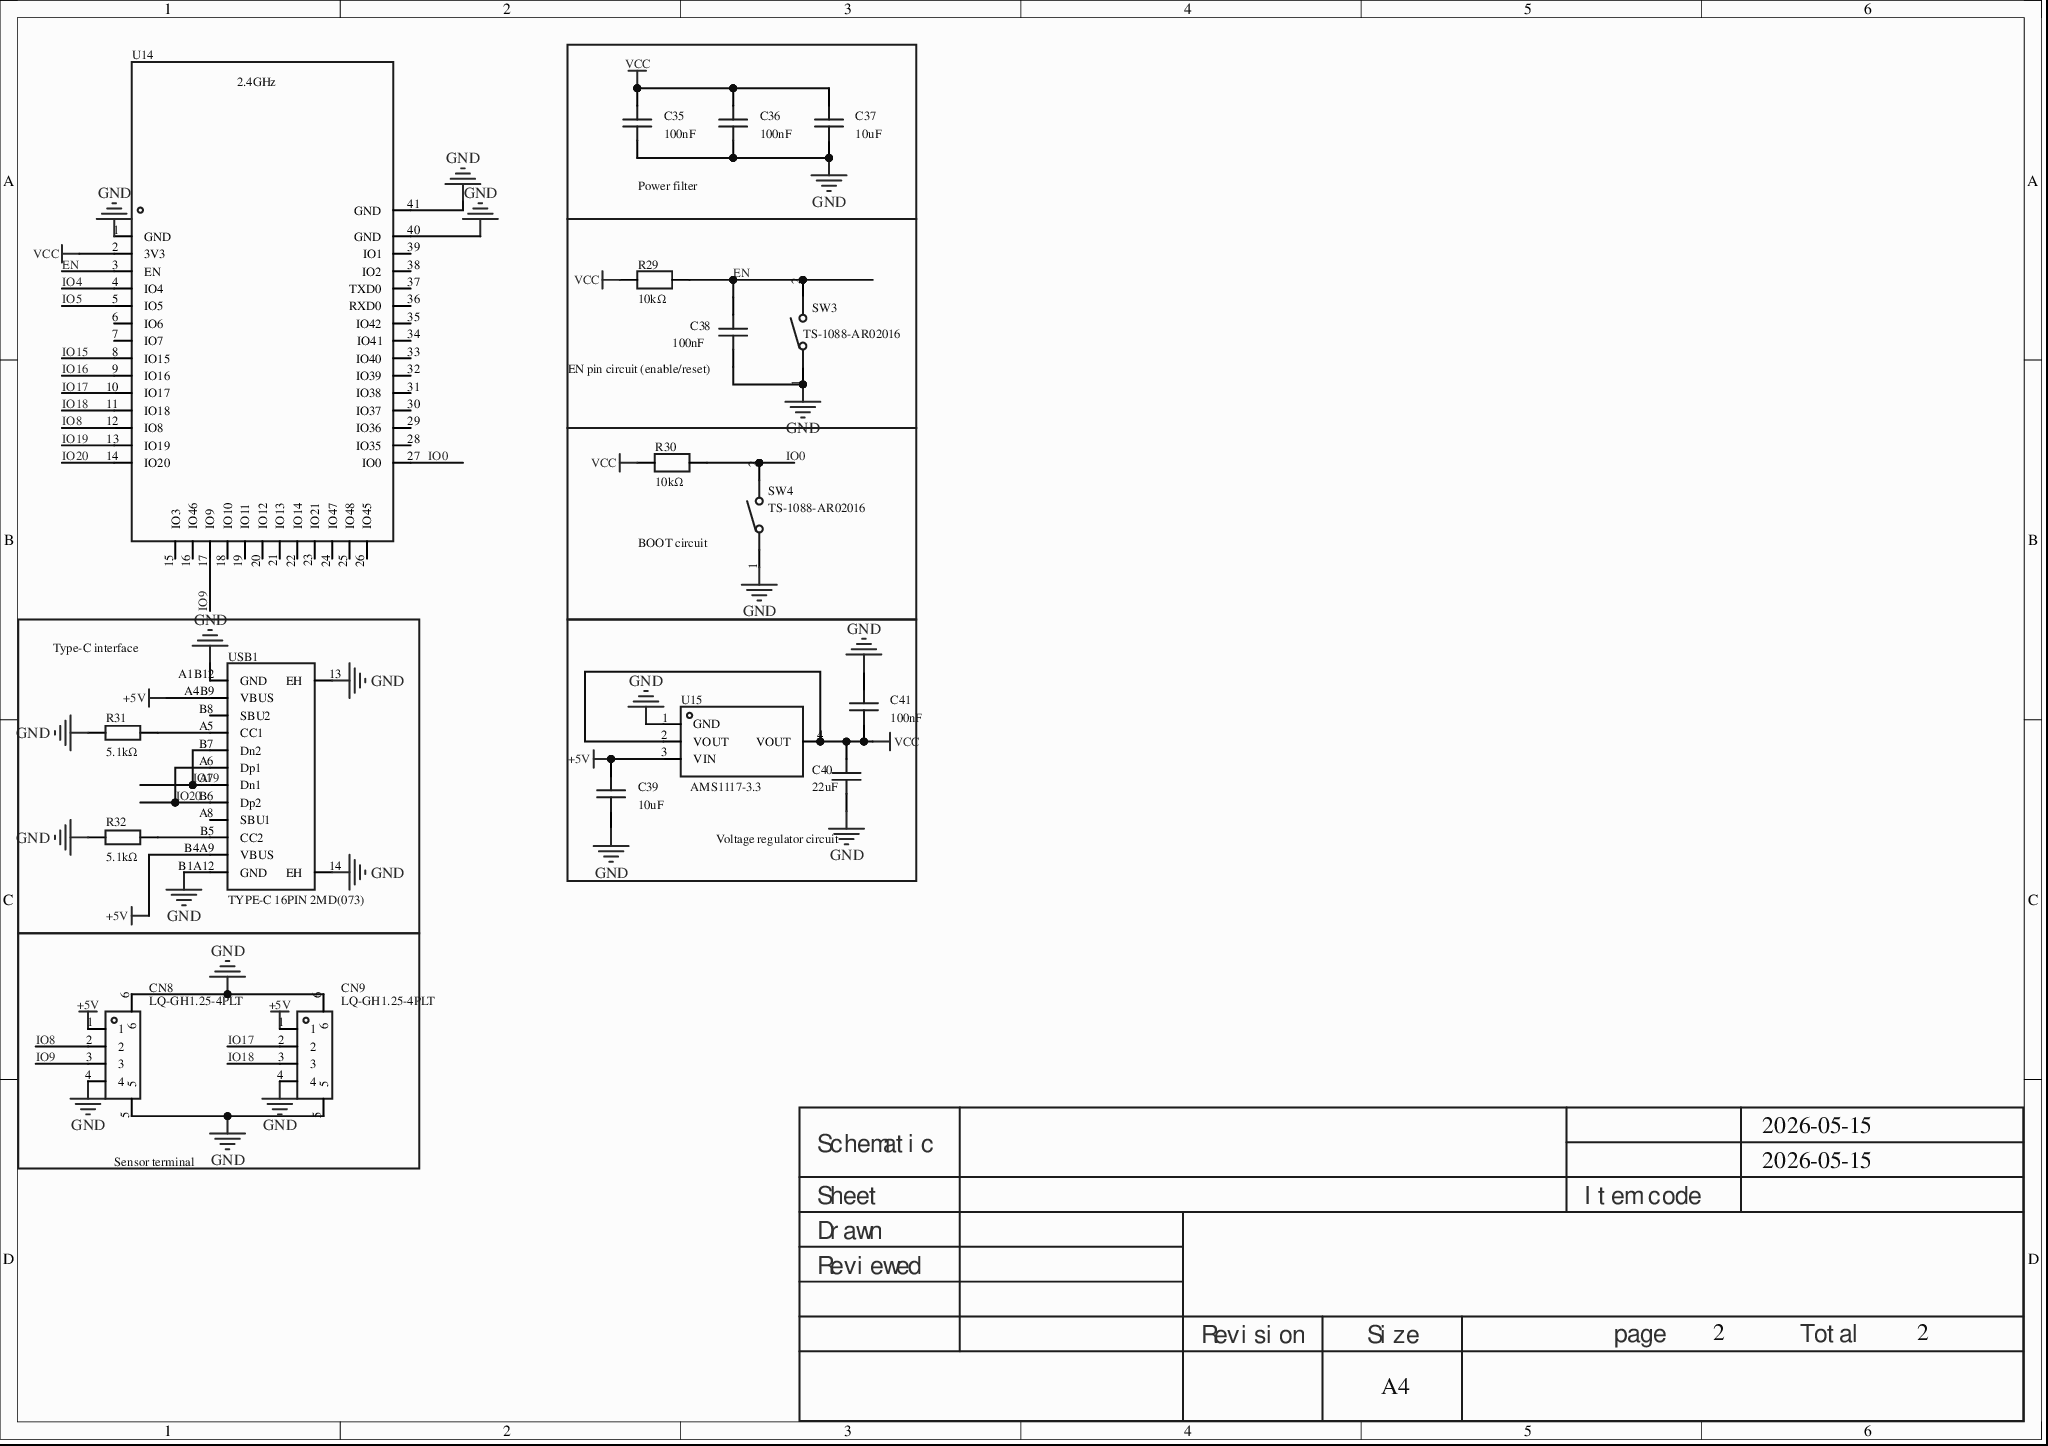
[diagram p0: MISC62500-3.schdoc]
# Altium project MISC62500-2.PrjPcb (part 1 of 2)
2 sheets, 106 parts. Net scope: global (net labels, ports and power ports of the same name join across sheets).
Board file: MISC62500.pcbdoc
Sheets:
  MISC62500-3.schdoc
  MISC62500-4.schdoc

## Sheet MISC62500-3.schdoc
size 297 x 209 mm; Version: V1.0; @Project Name: MISC62500; @Page Count: 2; @Update Date: 2026-05-15; @Create Date: 2026-05-15; @Schematic Name: MISC62500; @Page No: 2; @Board Name: MISC62500; @Create Time: 10:23:29; @Update Time: 19:47:53

### Parts
C35  100nF  [C0603]
C36  100nF  [C0603]
C37  10uF  [C0805]
C38  100nF  [C0603]
C39  10uF  [C0805]
C40  22uF  [C0805]
C41  100nF  [C0603]
CN8  LQ-GH1.25-4PLT  [CONN-SMD_LQ-GH1.25-4PLT]
CN9  LQ-GH1.25-4PLT  [CONN-SMD_LQ-GH1.25-4PLT]
R29  10kΩ  [R0603]
R30  10kΩ  [R0603]
R31  5.1kΩ  [R0603]
R32  5.1kΩ  [R0603]
SW3  TS-1088-AR02016  [SW-SMD_L3.9-W3.0-P4.45]
SW4  TS-1088-AR02016  [SW-SMD_L3.9-W3.0-P4.45]
U14  2.4GHz  [WIRELM-SMD_ESP32-S3-WROOM-1]
U15  AMS1117-3.3  [SOT-223-3_L6.5-W3.4-P2.30-LS7.0-BR]
USB1  TYPE-C 16PIN 2MD(073)  [USB-C-SMD_TYPE-C-16PIN-2MD-073]

### Blocks framed on the sheet
Power filter: C35-C37
EN pin circuit (enable/reset): C38 R29 SW3
BOOT circuit: R30 SW4
Type-C interface: R31 R32 USB1
Voltage regulator circuit: C39-C41 U15
Sensor terminal: CN8 CN9

### Nets
+5V: C39.2 CN8.1 CN9.1 U15.3(VIN) USB1.A4B9(VBUS) USB1.B4A9(VBUS)
GND: C35.1 C36.1 C37.1 C38.1 C39.1 C40.1 C41.2 CN8.4 CN8.5 CN8.6 CN9.4 CN9.5 CN9.6 R31.1 R32.1 SW3.1 SW4.1 U14.1(GND) U14.40(GND) U14.41(GND) U15.1(GND) USB1.13(EH) USB1.14(EH) USB1.A1B12(GND) USB1.B1A12(GND)
VCC: C35.2 C36.2 C37.2 C40.2 C41.1 R29.1 R30.1 U14.2(3V3) U15.2(VOUT) U15.4(VOUT)
EN: C38.2 R29.2 SW3.2 U14.3(EN)
IO0: R30.2 SW4.2 U14.27(IO0)
IO4: U14.4(IO4)
IO5: U14.5(IO5)
IO8: CN8.2 U14.12(IO8)
IO9: CN8.3 U14.17(IO9)
IO15: U14.8(IO15)
IO16: U14.9(IO16)
IO17: CN9.2 U14.10(IO17)
IO18: CN9.3 U14.11(IO18)
IO19: U14.13(IO19) USB1.A7(Dn1) USB1.B7(Dn2)
IO20: U14.14(IO20) USB1.A6(Dp1) USB1.B6(Dp2)
NetR31_2: R31.2 USB1.A5(CC1)
NetR32_2: R32.2 USB1.B5(CC2)

Not connected (* = marked no-connect by the designer): U14 6(IO6)* 7(IO7)* 15(IO3)* 16(IO46)* 18(IO10)* 19(IO11)* 20(IO12)* 21(IO13)* 22(IO14)* 23(IO21)* 24(IO47)* 25(IO48)* 26(IO45)* 28(IO35)* 29(IO36)* 30(IO37)* 31(IO38)* 32(IO39)* 33(IO40)* 34(IO41)* 35(IO42)* 36(RXD0)* 37(TXD0)* 38(IO2)* 39(IO1)*; USB1 A8(SBU1)* B8(SBU2)*

### Notes on the sheet
- 2026-05-15
- Schematic
- Sheet
- Item code
- Reviewed
- Drawn
- Revision
- Size
- A4
- page
- 2
- Total

### Library data of the parts
C35 C36 C38 C41 = CC0603KRX7R9BB104: Capacitance: 100nF; Tolerance: ±10%; Rated voltage: 50V; Temp coefficient: X7R;; Manufacturer: YAGEO(国巨); AddInBom: yes; ModelId: ac125912035d415993ca9572d50418b1; ModelName: C0603_L1.6-W0.8-H0.8; ModelTransform: 62.992,31.496,0,0,0,0,0,0,0; Symbol: CC0603KRX7R9BB104; Device: CC0603KRX7R9BB104; LCSC Part Name: 100nF ±10% 50V; SupplierPart: C14663; ManufacturerPart: CC0603KRX7R9BB104; Supplier Footprint: 0603; JLCPCB Part Class: Basic Part; Datasheet: example.com/datasheet/CC0603KRX7R9BB104/15331.html; Supplier: LCSC; ConvertToPcb: yes; FootprintName: C0603; Value: 100nF; Voltage Rating: 50V; Temperature Coefficient: X7R
C37 C39 = CGA0805X5R106K500MT: Capacitance: 10uF; Tolerance: ±10%; Rated voltage: 50V; Temp coefficient: X5R;; Manufacturer: HRE(芯声); AddInBom: yes; ModelId: 1ba041120af144c991958decab20d241; ModelName: C0805_L2.0-W1.3-H1.3; ModelTransform: 78.74,51.181,0,0,0,0,0,0.0005,0; Symbol: CGA0805X5R106K500MT; Device: CGA0805X5R106K500MT; LCSC Part Name: 10uF ±10% 50V; SupplierPart: C6119889; ManufacturerPart: CGA0805X5R106K500MT; Supplier Footprint: 0805; JLCPCB Part Class: Extended Part; Datasheet: example.com/datasheet/CGA0805X5R106K500MT/7062595.html; Supplier: LCSC; ConvertToPcb: yes; FootprintName: C0805; Value: 10uF; Voltage Rating: 50V; Temperature Coefficient: X5R
C40 = CGA0805X5R226M350MT: Capacitance: 22uF; Tolerance: ±20%; Rated voltage: 35V; Temp coefficient: X5R;; Manufacturer: HRE(芯声); AddInBom: yes; ModelId: 1ba041120af144c991958decab20d241; ModelName: C0805_L2.0-W1.3-H1.3; ModelTransform: 78.74,51.181,0,0,0,0,0,0.0005,0; Symbol: CGA0805X5R226M350MT; Device: CGA0805X5R226M350MT; LCSC Part Name: 22uF ±20% 35V; SupplierPart: C6119901; ManufacturerPart: CGA0805X5R226M350MT; Supplier Footprint: 0805; JLCPCB Part Class: Extended Part; Datasheet: example.com/datasheet/CGA0805X5R226M350MT/7062607.html; Supplier: LCSC; ConvertToPcb: yes; FootprintName: C0805; Value: 22uF; Voltage Rating: 35V; Temperature Coefficient: X5R
CN8 CN9 = LQ-GH1.25-4PLT: 1.25mm pitch 1x4P vertical-exit SMD wire-to-board header, suitable for SMT reflow; Manufacturer: LINGQIANG(领强); AddInBom: yes; Symbol: LQ-GH1.25-4PLT; Device: LQ-GH1.25-4PLT; LCSC Part Name: GH1.25立贴4P冷封盘; SupplierPart: C54618758; ManufacturerPart: LQ-GH1.25-4PLT; Supplier Footprint: SMD,P=1.25mm; JLCPCB Part Class: Extended Part; Datasheet: example.com/datasheet/LQ-GH1.25-4PLT/58013283.html; Supplier: LCSC; ConvertToPcb: yes; FootprintName: CONN-SMD_LQ-GH1.25-4PLT
R29 R30 = FRC0603F1002TS: Resistor type: thick film resistor; Resistance: 10kΩ; Tolerance: ±1%; Power: 100mW; Working voltage: 75V; Temp coefficient: ±100ppm/℃;; Manufacturer: FOJAN(富捷); AddInBom: yes; ModelId: fc143cca1e79419f9cd78b61e9279f08; ModelTransform: 31.8897,63.7794,0,90,0,0,0,0,0; Symbol: FRC0603F1002TS; Device: FRC0603F1002TS; LCSC Part Name: 10kΩ ±1% 100mW 厚膜电阻; SupplierPart: C2906982; ManufacturerPart: FRC0603F1002TS; Supplier Footprint: 0603; JLCPCB Part Class: Extended Part; Supplier: LCSC; ConvertToPcb: yes; FootprintName: R0603; ModelName: R0603; Type: Thick film resistor; Value: 10kΩ; Power(Watts): 100mW; Voltage-Supply(Max): 75V; Temperature Coefficient: ±100ppm/℃; Operating Temperature: -55℃~+155℃
R31 R32 = 0603WAF5101T5E: Resistor type: thick film resistor; Resistance: 5.1kΩ; Tolerance: ±1%; Power: 100mW; Working voltage: 75V; Temp coefficient: ±100ppm/℃;; Manufacturer: UNI-ROYAL(厚声); AddInBom: yes; ModelId: fc143cca1e79419f9cd78b61e9279f08; ModelTransform: 31.8897,63.7794,0,90,0,0,0,0,0; Symbol: 0603WAF5101T5E; Device: 0603WAF5101T5E; LCSC Part Name: 5.1kΩ ±1% 100mW 厚膜电阻; SupplierPart: C23186; ManufacturerPart: 0603WAF5101T5E; Supplier Footprint: 0603; JLCPCB Part Class: Basic Part; Datasheet: example.com/datasheet/0603WAF5101T5E/23913.html; Supplier: LCSC; ConvertToPcb: yes; FootprintName: R0603; ModelName: R0603; Type: Thick film resistor; Value: 5.1kΩ; Power(Watts): 100mW; Voltage-Supply(Max): 75V; Temperature Coefficient: ±100ppm/℃; Operating Temperature: -55℃~+155℃
SW3 SW4 = TS-1088-AR02016: 电路结构:单刀单掷;按钮形状:圆形按钮;作用力:1.6N;安装方式:立贴;开关长度:4mm;开关宽度:3mm;开关高度:2mm;带支架:不带支架;触点电流:50mA;额定电压:12V;工作寿命:10万次;; Manufacturer: XUNPU(讯普); AddInBom: yes; ModelId: b26698b69f274ffabef8a26c7d0e5dd1; ModelName: SW-SMD_L3.9-W2.9-H2.0-LS4.8; ModelTransform: 188.976,114.174,0,0,0,0,0,0,0; Circuit: SPST; Actuator Style: Round button; Operating Force: 1.6N; Switch Height: 2mm; with Bracket: Without bracket; Contact Current: 50mA; Voltage Rating: 12V; Actuator/Cap Color: Black; Life: 10 x 10k cycles; Symbol: TS-1088-AR02016; Device: TS-1088-AR02016; LCSC Part Name: 4*3*2mm 立贴 轻触开关; SupplierPart: C720477; ManufacturerPart: TS-1088-AR02016; Supplier Footprint: SMD,4x3mm; JLCPCB Part Class: Basic Part; Datasheet: example.com/datasheet/TS-1088-AR02016/763484.html; Supplier: LCSC; ConvertToPcb: yes; FootprintName: SW-SMD_L3.9-W3.0-P4.45; Mounting Type: Vertical SMD; Length: 4mm; Width: 3mm; Termination Style: SMD tab; Operating Temperature: -30℃~+80℃
U14 = ESP32-S3-WROOM-1-N16R8: Core chip: ESP32-S3R8; Frequency: 2.4GHz; Antenna: on-board PCB antenna; TX power: 20.5dBm; RX sensitivity: -103.5dBm;; Manufacturer: ESPRESSIF(乐鑫); Symbol: ESP32-S3-WROOM-1(N16R8); AddInBom: yes; ModelId: 481f5bdfc076422c9bb3c23c3ada9c17; ModelTransform: 708.73866,1003.97437,0,0,0,0,0,143.7,0; Interface Type: I2C; GPIO; UART; SPI; USB; I2S; Voltage - Supply: 3V~3.6V; Receive  Current: 95mA; Send  Current: 355mA; Device: ESP32-S3-WROOM-1-N16R8; LCSC Part Name: 不带固件 通用型Wi-Fi+低功耗蓝牙MCU模组; SupplierPart: C2913202; ManufacturerPart: ESP32-S3-WROOM-1-N16R8; Supplier Footprint: SMD,25.5x18mm; JLCPCB Part Class: Extended library; Datasheet: example.com/datasheet/ESP32-S3-WROOM-1-N16R8/3198300.html; Supplier: LCSC; ConvertToPcb: yes; FootprintName: WIRELM-SMD_ESP32-S3-WROOM-1; ModelName: WIRELM-SMD_ESP32-S3-WROOM-1; Utilized IC / Part: ESP32-S3R8; Value: 2.4GHz; Antenna Type: On-board PCB antenna; Output Power: 20.5dBm; Sensitivity: -103.5dBm; Operating Temperature: -40℃~+65℃
U15 = AMS1117-3.3_C6186: Output type: fixed; Working voltage: 15V; Output voltage: 3.3V; Output current: 1A; PSRR: 72dB@(120Hz); Output polarity: positive;; Manufacturer: AMS; AddInBom: yes; ModelId: 925194bf9823436183a3e0b978a8d076; ModelName: SOT-223-4P_L6.5-W3.5-H1.6-LS7.0-P2.30; ModelTransform: 279.89794,255.905,0,180,0,0,-3.9385,-0.0005,0; Voltage Dropout: 1.1V@(800mA); standby current: 5mA; Noise: 0.003%Vout; Number of Outputs: 1; Symbol: AMS1117-3.3; Device: AMS1117-3.3_C6186; LCSC Part Name: 3.3V 1A 15V; SupplierPart: C6186; ManufacturerPart: AMS1117-3.3; Supplier Footprint: SOT-223; JLCPCB Part Class: Basic Part; Datasheet: example.com/datasheet/AMS1117-3.3/6652.html; Supplier: LCSC; ConvertToPcb: yes; FootprintName: SOT-223-3_L6.5-W3.4-P2.30-LS7.0-BR; Output Type: Fixed; Voltage - Supply: 15V; Output Voltage: 3.3V; Output Current: 1A; Power Supply Rejection Ratio (PSRR): 72dB@(120Hz); Features: Overcurrent protection; thermal shutdown; Operating Temperature: -40℃~+125℃; Output Configuration: Positive
USB1 = TYPE-C 16PIN 2MD(073): Connector type: Type-C; Protocol standard: -; Gender: Female; Mounting: Flat SMD; Contacts: 16P; Ports: 1; Rated current - power: 3A; Operating temp: -25℃~+85℃;; Manufacturer: SHOU HAN(首韩); AddInBom: yes; ModelId: 3a41b9ec9b654a0fad4d118405ec6290; ModelName: USB-C-SMD_TYPE-C-6PIN-2MD-073; ModelTransform: 351.9678,298.4246,0,0,0,0,0,-47.244,-35.433; Number of Ports: 1; Voltage Rating: 5V; Connect-Disconnect Life: 1 x 10k cycles; Detection color: Black; Symbol: TYPE-C 16PIN 2MD(073); Device: TYPE-C 16PIN 2MD(073); LCSC Part Name: Type-C 母 卧贴; SupplierPart: C2765186; ManufacturerPart: TYPE-C 16PIN 2MD(073); Supplier Footprint: SMD; JLCPCB Part Class: Extended Part; Datasheet: example.com/datasheet/TYPE-C%252016PIN%25202MD(073)/2901843.html; Supplier: LCSC; ConvertToPcb: yes; FootprintName: USB-C-SMD_TYPE-C-16PIN-2MD-073; Connector Type: Type-C; Protocol Standard: -; Mounting Type: Flat SMD; Number of Contacts: 16P; Current Rating-Power: 3A; Supplementary Features: -; Center Height: -; Length: -; Operating Temperature: -25℃~+85℃

## Sheet MISC62500-4.schdoc
size 178 x 98 mm; Version: V1.0; @Project Name: MISC62500; @Page Count: 2; @Update Date: 2026-05-12; @Create Date: 2026-05-12; @Schematic Name: MISC62500; @Page No: 1; @Board Name: MISC62500; @Create Time: 10:47:24; @Update Time: 15:30:59
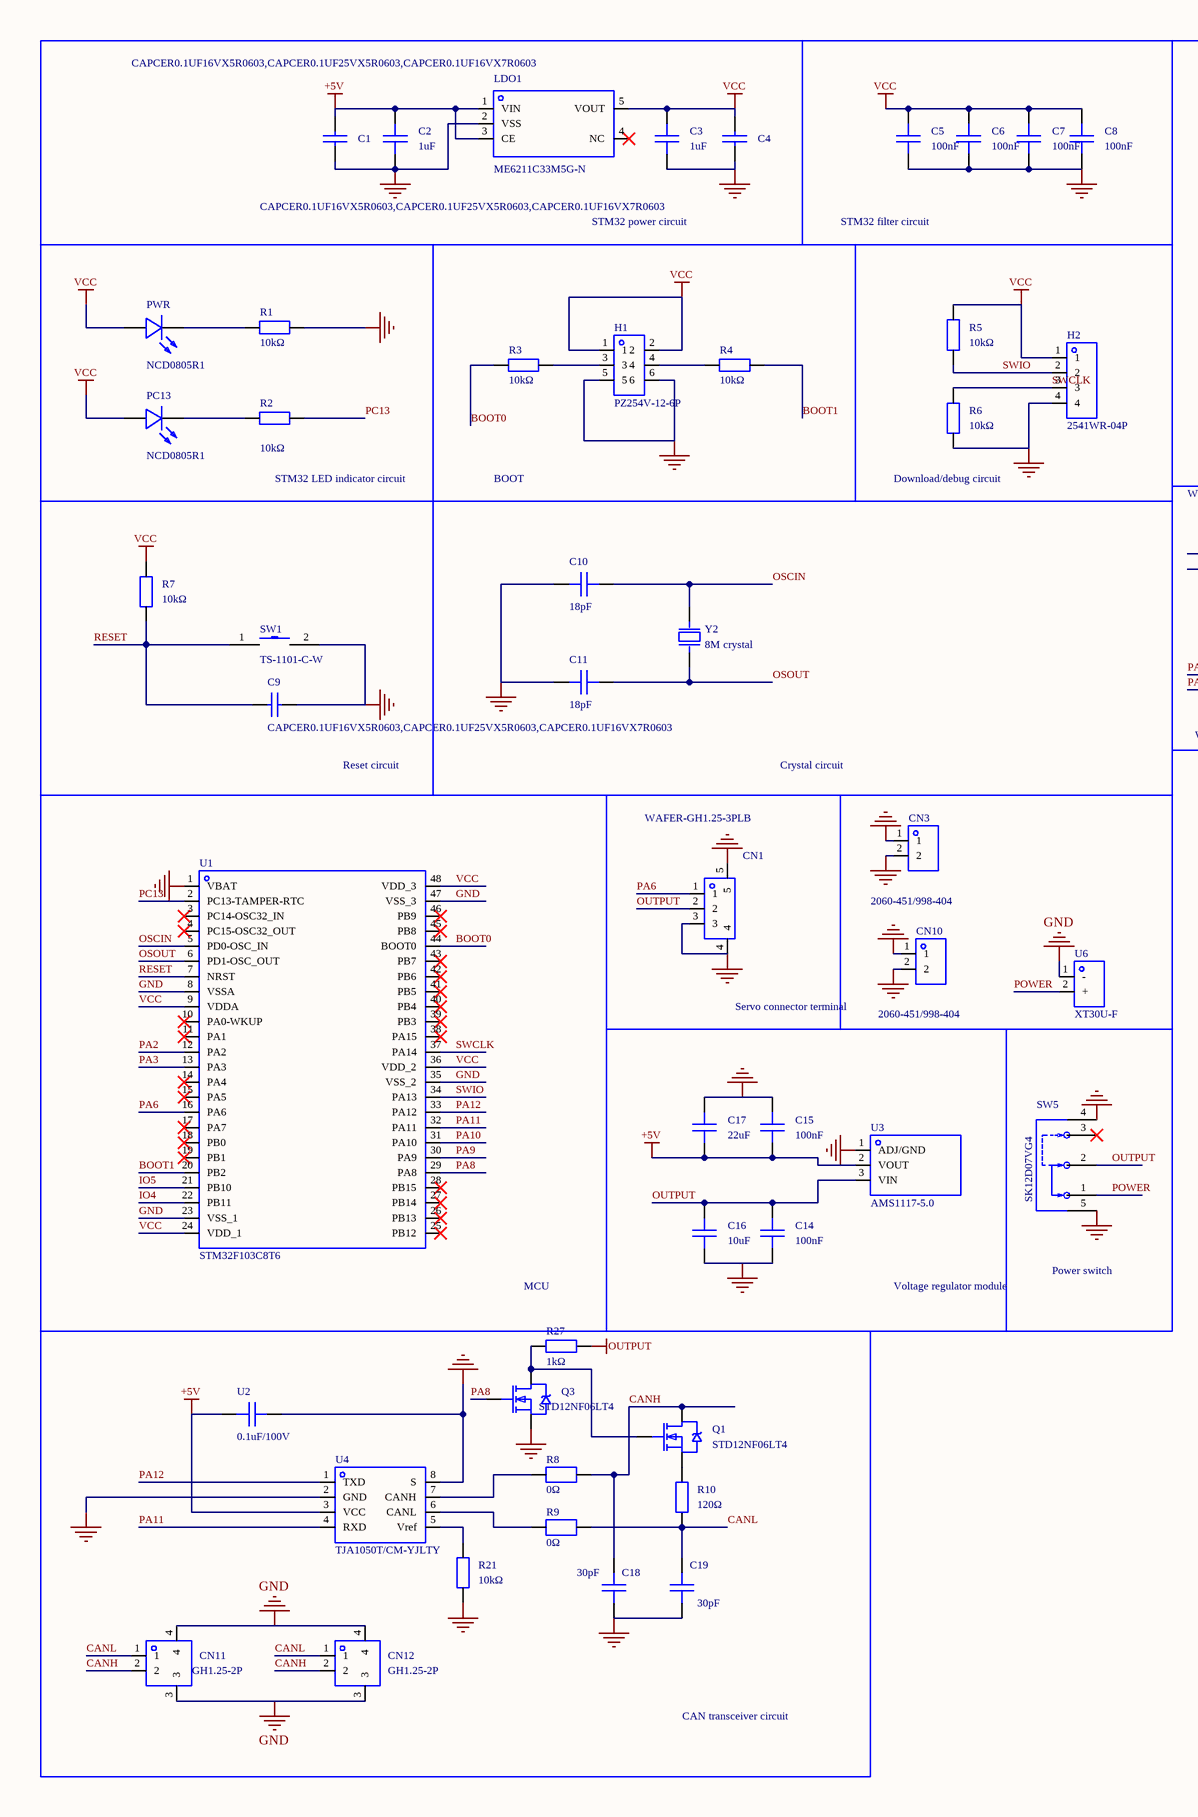
[diagram p1: MISC62500-4.schdoc, left]
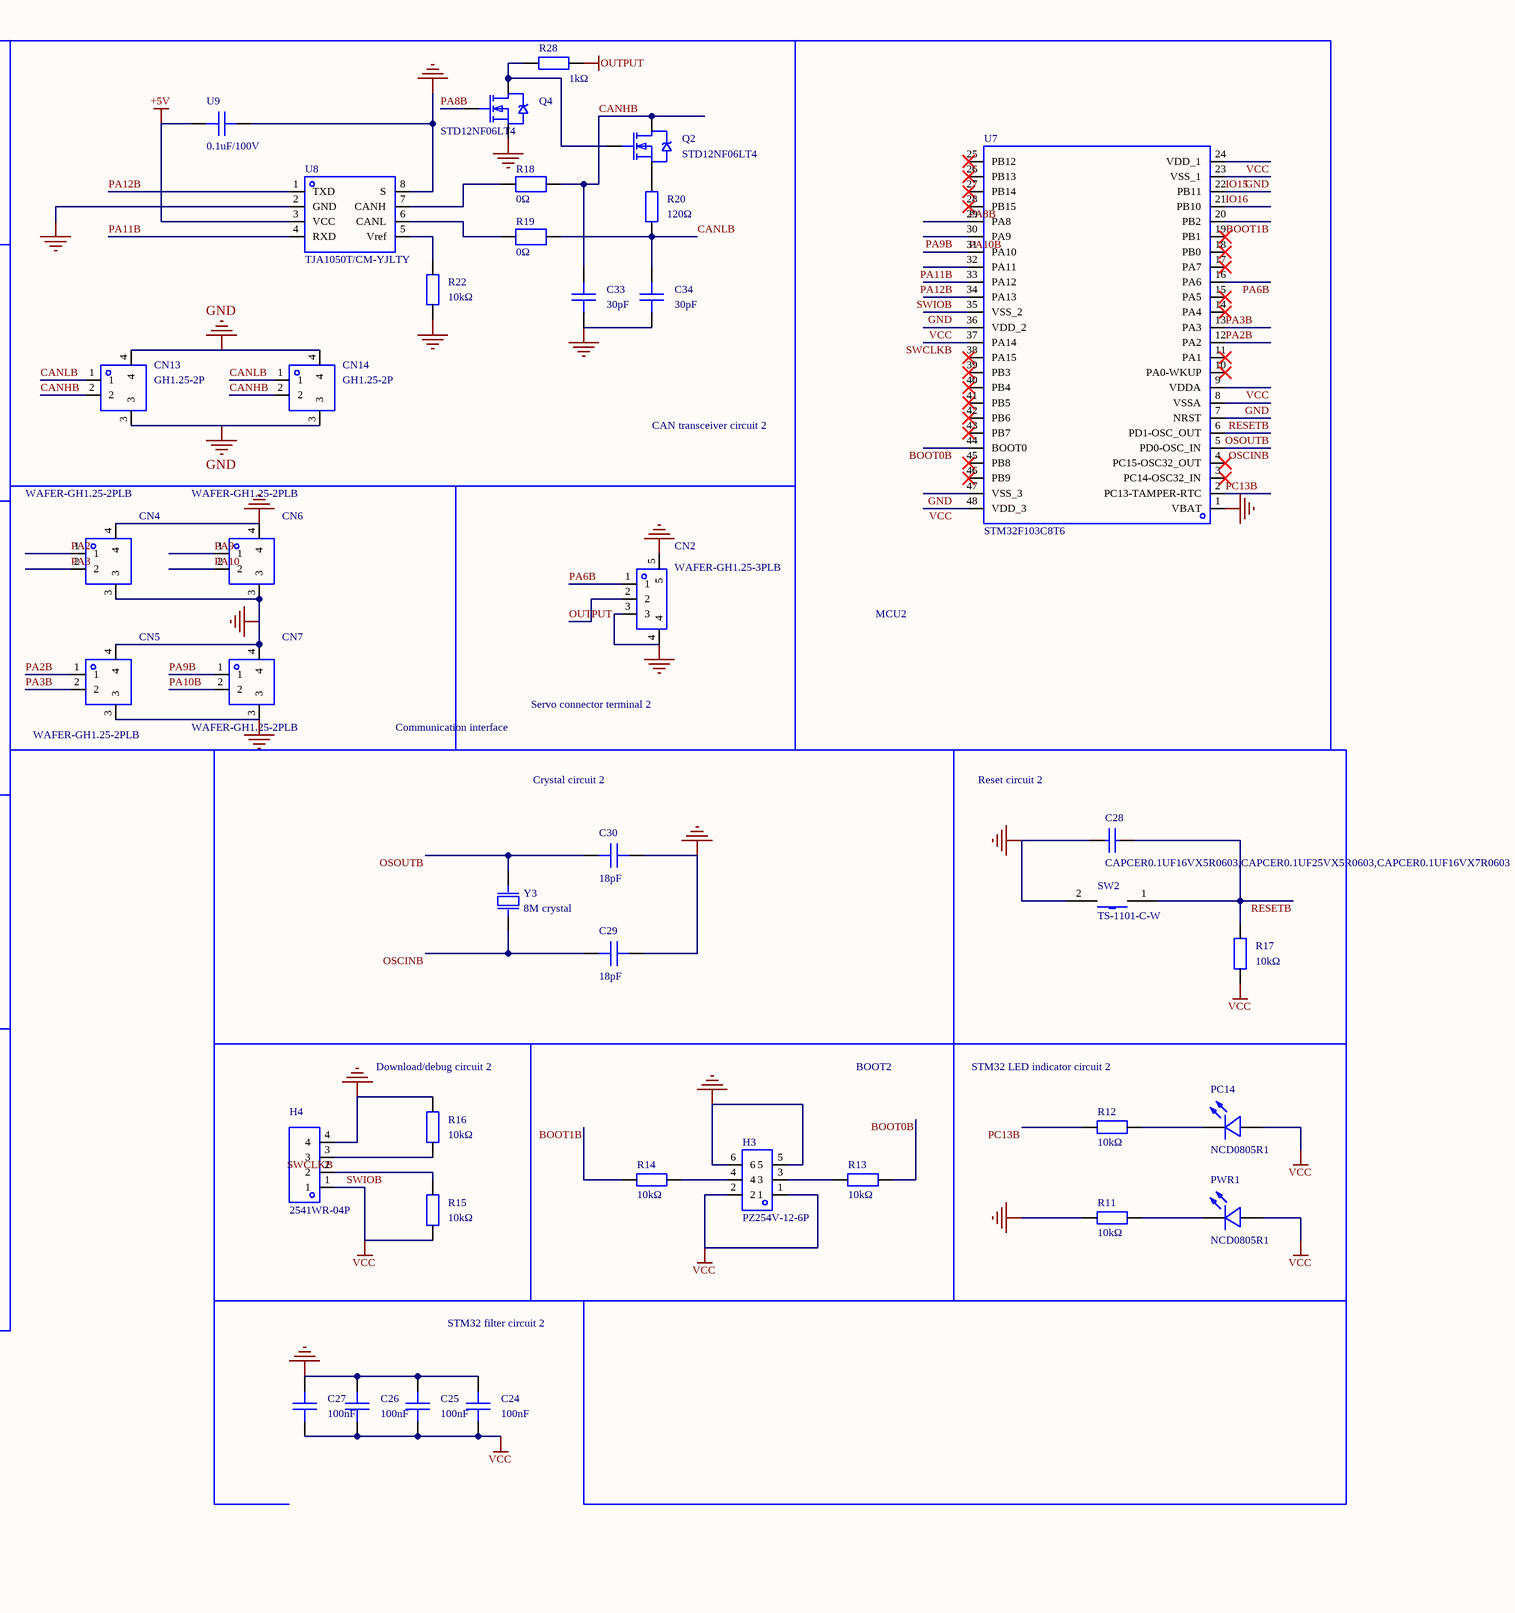
[diagram p2: MISC62500-4.schdoc, right]

### Parts
C1  CAPCER0.1UF16VX5R0603,CAPCER0.1UF25VX5R0603,CAPCER0.1UF16VX7R0603  [C0603]
C2  1uF  [C0603]
C3  1uF  [C0603]
C4  CAPCER0.1UF16VX5R0603,CAPCER0.1UF25VX5R0603,CAPCER0.1UF16VX7R0603  [C0603]
C5  100nF  [C0603]
C6  100nF  [C0603]
C7  100nF  [C0603]
C8  100nF  [C0603]
C9  CAPCER0.1UF16VX5R0603,CAPCER0.1UF25VX5R0603,CAPCER0.1UF16VX7R0603  [C0603]
C10  18pF  [C0603]
C11  18pF  [C0603]
C14  100nF  [C0603]
C15  100nF  [C0603]
C16  10uF  [C0603]
C17  22uF  [C0603]
C18  30pF  [C0805]
C19  30pF  [C0805]
C24  100nF  [C0603]
C25  100nF  [C0603]
C26  100nF  [C0603]
C27  100nF  [C0603]
C28  CAPCER0.1UF16VX5R0603,CAPCER0.1UF25VX5R0603,CAPCER0.1UF16VX7R0603  [C0603]
C29  18pF  [C0603]
C30  18pF  [C0603]
C33  30pF  [C0805]
C34  30pF  [C0805]
CN1  WAFER-GH1.25-3PLB  [CONN-SMD_3P-P1.25_XUNPU_WAFER-GH1.25-3PLB]
CN2  WAFER-GH1.25-3PLB  [CONN-SMD_3P-P1.25_XUNPU_WAFER-GH1.25-3PLB]
CN3  2060-451/998-404  [CONN-SMD_L12.7-W3.9_2060-451-998-404]
CN4  WAFER-GH1.25-2PLB  [CONN-TH_2P-P1.25_XUNPU_WAFER-GH1.25-2PLB]
CN5  WAFER-GH1.25-2PLB  [CONN-TH_2P-P1.25_XUNPU_WAFER-GH1.25-2PLB]
CN6  WAFER-GH1.25-2PLB  [CONN-TH_2P-P1.25_XUNPU_WAFER-GH1.25-2PLB]
CN7  WAFER-GH1.25-2PLB  [CONN-TH_2P-P1.25_XUNPU_WAFER-GH1.25-2PLB]
CN10  2060-451/998-404  [CONN-SMD_L12.7-W3.9_2060-451-998-404]
CN11  GH1.25-2P  [CONN-TH_2P-P1.25_XUNPU_WAFER-GH1.25-2PLB]
CN12  GH1.25-2P  [CONN-TH_2P-P1.25_XUNPU_WAFER-GH1.25-2PLB]
CN13  GH1.25-2P  [CONN-TH_2P-P1.25_XUNPU_WAFER-GH1.25-2PLB]
CN14  GH1.25-2P  [CONN-TH_2P-P1.25_XUNPU_WAFER-GH1.25-2PLB]
H1  PZ254V-12-6P  [HDR-TH_6P-P2.54-V-M-R2-C3-S2.54]
H2  2541WR-04P  [HDR-TH_4P-P2.54-H-M-W10.4-N]
H3  PZ254V-12-6P  [HDR-TH_6P-P2.54-V-M-R2-C3-S2.54]
H4  2541WR-04P  [HDR-TH_4P-P2.54-H-M-W10.4-N]
LDO1  ME6211C33M5G-N  [SOT-23-5_L3.0-W1.7-P0.95-LS2.8-BL]
PC13  NCD0805R1  [LED0805-R-RD]
PC14  NCD0805R1  [LED0805-R-RD]
PWR  NCD0805R1  [LED0805-R-RD]
PWR1  NCD0805R1  [LED0805-R-RD]
Q1  STD12NF06LT4  [TO-252-3_L6.5-W5.8-P4.58-BL]